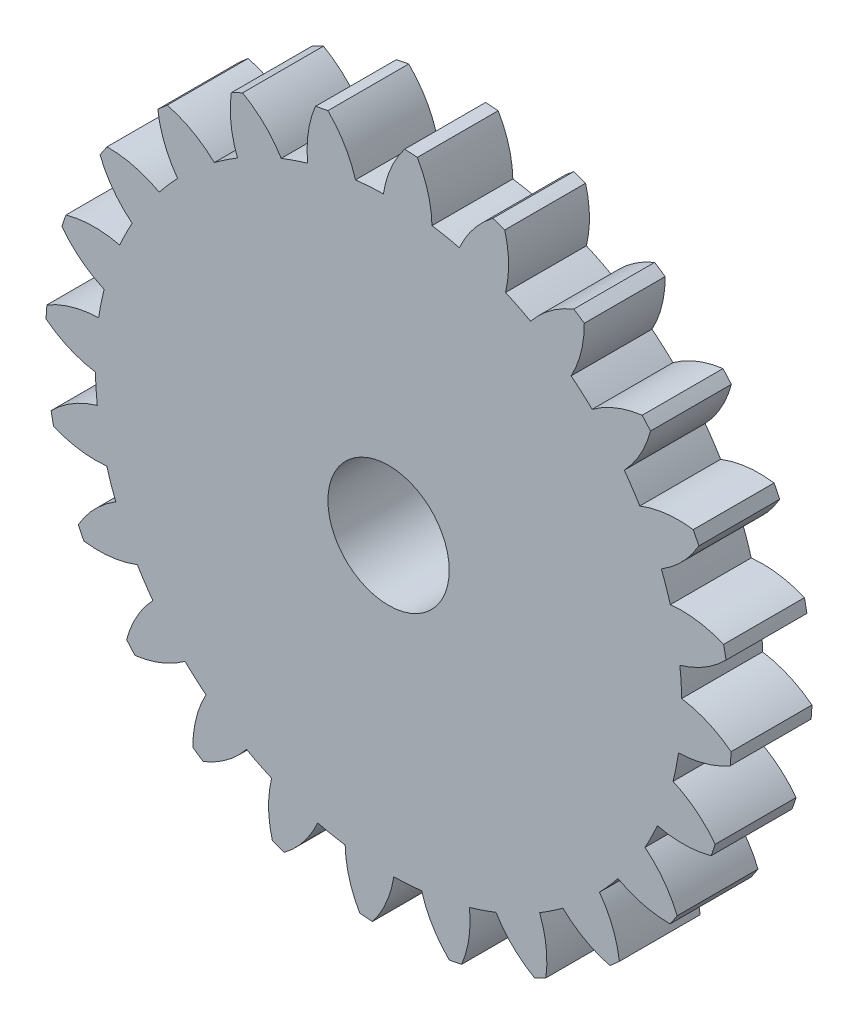
SolidWorks part; units mm, degrees
ref_plane "Front Plane" through (0, 0, 0) normal (0, 0, 1) x (1, 0, 0)
ref_plane "Top Plane" through (0, 0, 0) normal (0, 1, 0) x (1, 0, 0)
ref_plane "Right Plane" through (0, 0, 0) normal (1, 0, 0) x (0, 0, -1)
sketch "Sketch1" plane through (0, 0, 0) normal (0, 0, 1) x (1, 0, 0)
  circle A0 centre (0, 0) radius 7.25
  dimension "D1" = 14.5
extrude "Boss-Extrude1" add sketch "Sketch1" along normal blind 2
sketch "Sketch2" plane through (0, 0, 2) normal (0, 0, 1) x (1, 0, 0)
  line L0 (0, 0) -> (0, 12.6742) construction
  line L1 (0, 0) -> (4.4384, 12.1945) construction
  line L2 (0, 0) -> (0.8307, 12.6743) construction
  line L3 (0, 7.75) -> (2.4908, 6.8434) construction
  circle A0 centre (0, 0) radius 7.75 construction
  arc A1 (0.7106, 8.4502) -> (0.3984, 8.4706) centre (0, 0) ccw
  arc A2 (0.3984, 8.4706) -> (-0.1582, 6.9374) centre (2.4908, 6.8434) ccw
  arc A4 (0.7106, 8.4502) -> (1.0623, 6.8574) centre (-1.5762, 7.11) cw
  arc A5 (1.0623, 6.8574) -> (-0.1582, 6.9374) centre (0, 0) ccw
  dimension "D1" = 15.5
  dimension "D2" = 16.96
  dimension "D3" = 20
  dimension "D4" = 3.75
sketch "Sketch3" plane through (0, 0, 0) normal (0, 0, -1) x (-1, 0, 0)
  circle A0 centre (0, 0) radius 4.7062
ref_plane "Plane1" through (0, 0, -0.8) normal (0, 0, -1) x (-1, 0, 0)
sketch "Sketch4" plane through (0, 0, -0.8) normal (0, 0, -1) x (-1, 0, 0)
  circle A0 centre (0, 0) radius 2.4207
loft "Loft1" add profiles "Sketch3", "Sketch4"
sketch "Sketch5" plane through (0, 0, -0.8) normal (0, 0, -1) x (-1, 0, 0)
  circle A0 centre (0, 0) radius 2.4207
extrude "Boss-Extrude3" add sketch "Sketch5" along normal blind 1
fillet "Fillet1" radius 0.3 2 edges at (-2.4207, 0, -0.8) (-2.4207, 0, -1.8)
extrude "Boss-Extrude4" add sketch "Sketch2" against normal up to surface (2 mm away) up to face at (-4.7062, 0, 0)
pattern_circular "CirPattern2" count 24 over 360 about axis through (0, 0, 0) along (0, 0, 1) of "Boss-Extrude4"
sketch "Sketch6" plane through (0, 0, -1.8) normal (0, 0, -1) x (-1, 0, 0)
  circle A0 centre (0, 0) radius 1.5
  dimension "D1" = 3
extrude "Cut-Extrude1" cut sketch "Sketch6" against normal blind 10
